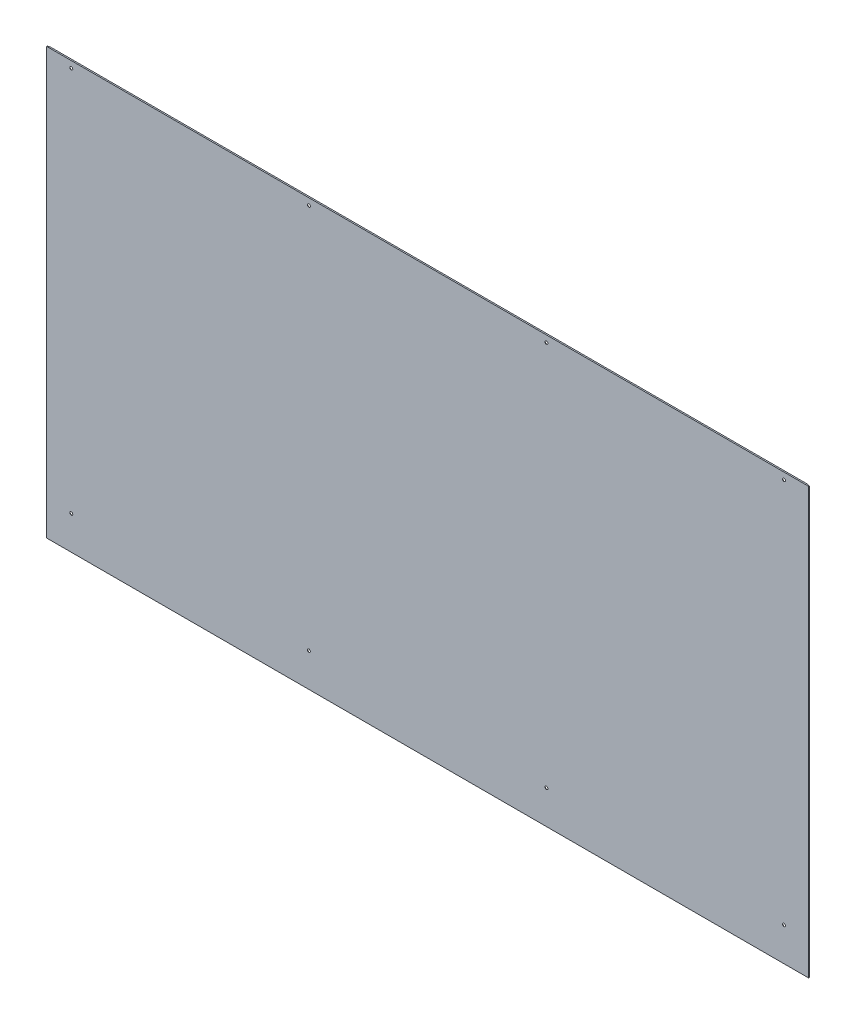
SolidWorks part; units mm, degrees
material "1023 碳钢板 (SS)"
ref_plane "前视基准面" through (0, 0, 0) normal (0, 0, 1) x (1, 0, 0)
ref_plane "上视基准面" through (0, 0, 0) normal (0, 1, 0) x (1, 0, 0)
ref_plane "右视基准面" through (0, 0, 0) normal (1, 0, 0) x (0, 0, -1)
sketch "草图1" plane through (0, 0, 0) normal (0, 0, 1) x (1, 0, 0)
  line L1 (-850, 475) -> (850, 475)
  line L2 (-850, 475) -> (-850, -475)
  line L3 (-850, -475) -> (850, -475)
  line L4 (850, 475) -> (850, -475)
  line L5 (-850, 475) -> (850, -475) construction
  line L6 (-850, -475) -> (850, 475) construction
  point P0 (0, 0)
  dimension "D1" = 1700
  dimension "D2" = 950
extrude "凸台-拉伸1" add sketch "草图1" along normal blind 3
sketch "草图2" plane through (0, 0, 3) normal (0, 0, 1) x (1, 0, 0)
  line L0 (850, 475) -> (-850, 475) construction
  line L1 (-795, 460) -> (795, 460) construction
  line L2 (-795, 460) -> (-795, -400) construction
  line L3 (-795, -400) -> (795, -400) construction
  line L4 (795, 460) -> (795, -400) construction
  line L7 (-850, 475) -> (-850, -475) construction
  line L8 (-265, 460) -> (-265, -400) construction
  line L9 (265, 460) -> (265, -400) construction
  circle A0 centre (-795, 460) radius 3.25
  circle A1 centre (-265, 460) radius 3.25
  circle A2 centre (265, 460) radius 3.25
  circle A3 centre (795, 460) radius 3.25
  circle A4 centre (795, -400) radius 3.25
  circle A5 centre (265, -400) radius 3.25
  circle A6 centre (-265, -400) radius 3.25
  circle A7 centre (-795, -400) radius 3.25
  point P0 (0, 0)
  dimension "D7" = 6.5
  dimension "D1" = 860
  dimension "D2" = 15
  dimension "D3" = 55
  dimension "D4" = 530
  dimension "D5" = 530
  dimension "D6" = 530
extrude "切除-拉伸1" cut sketch "草图2" against normal blind 3 draft 45 draft outward yes
sketch "草图3" plane through (0, -475, 0) normal (0, -1, 0) x (1, 0, 0)
  line L0 (844.4019, 0) -> (850, 1.5)
  line L1 (850, 0) -> (-850, 0) construction
  line L5 (850, 3) -> (850, 0) construction
  line L6 (850, 1.5) -> (850, 0)
  line L7 (850, 0) -> (844.4019, 0)
  line L8 (0, 0) -> (0, 11.2824) construction
  line L9 (-850, 1.5) -> (-850, 0)
  line L10 (-850, 0) -> (-844.4019, 0)
  line L11 (-844.4019, 0) -> (-850, 1.5)
  dimension "D1" = 15
  dimension "D2" = 1.5
extrude "切除-拉伸2" cut sketch "草图3" against normal through all contours L9 L10 L11 | L0 L6 L7
